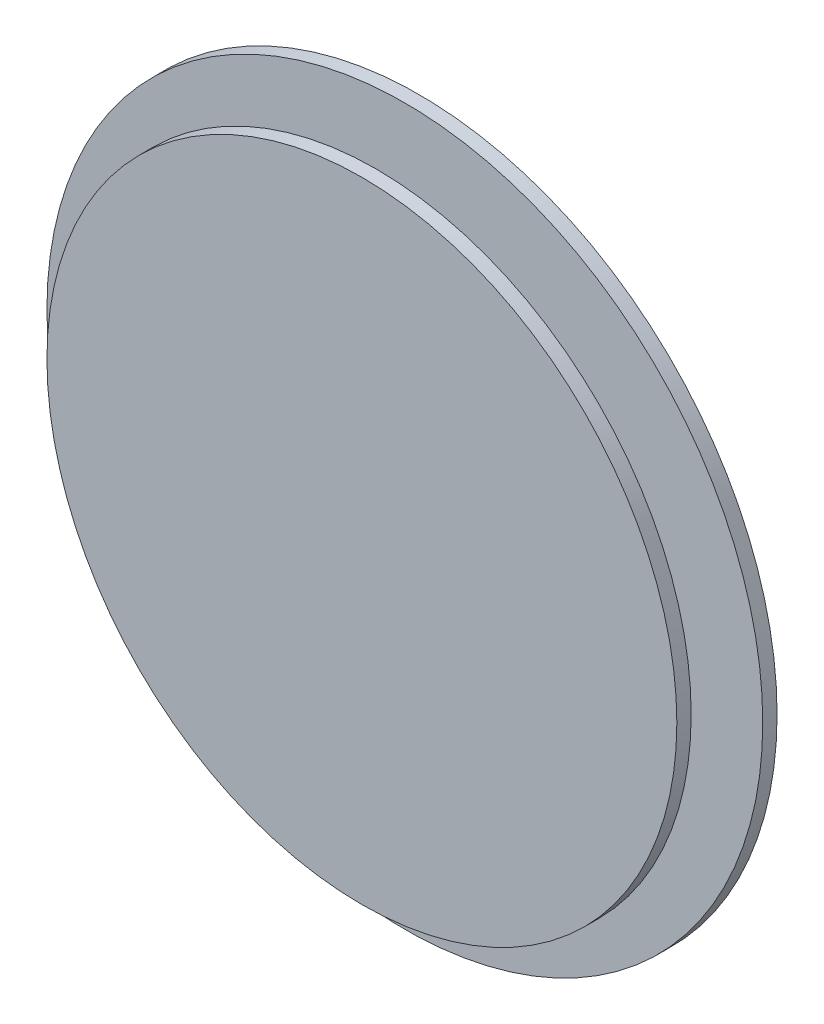
SolidWorks part; units mm, degrees
ref_plane "Front plane" through (0, 0, 0) normal (0, 0, 1) x (1, 0, 0)
ref_plane "Top plane" through (0, 0, 0) normal (0, 1, 0) x (1, 0, 0)
ref_plane "Right plane" through (0, 0, 0) normal (1, 0, 0) x (0, 0, -1)
sketch "Sketch 3" plane through (0, 0, 0) normal (0, 0, 1) x (1, 0, 0)
  circle A0 centre (0, 0) radius 25
  dimension "D1" = 50
extrude "Boss-Extrude 1" add sketch "Sketch 3" along normal blind 1
sketch "Sketch 4" plane through (0, 0, 1) normal (0, 0, 1) x (1, 0, 0)
  circle A0 centre (0, 0) radius 19
  dimension "D1" = 38
extrude "Boss-Extrude 2" add sketch "Sketch 4" along normal blind 2
sketch "Sketch 5" plane through (0, 0, 3) normal (0, 0, 1) x (1, 0, 0)
  circle A0 centre (0, 0) radius 22
  dimension "D1" = 44
extrude "Boss-Extrude 3" add sketch "Sketch 5" along normal blind 1
